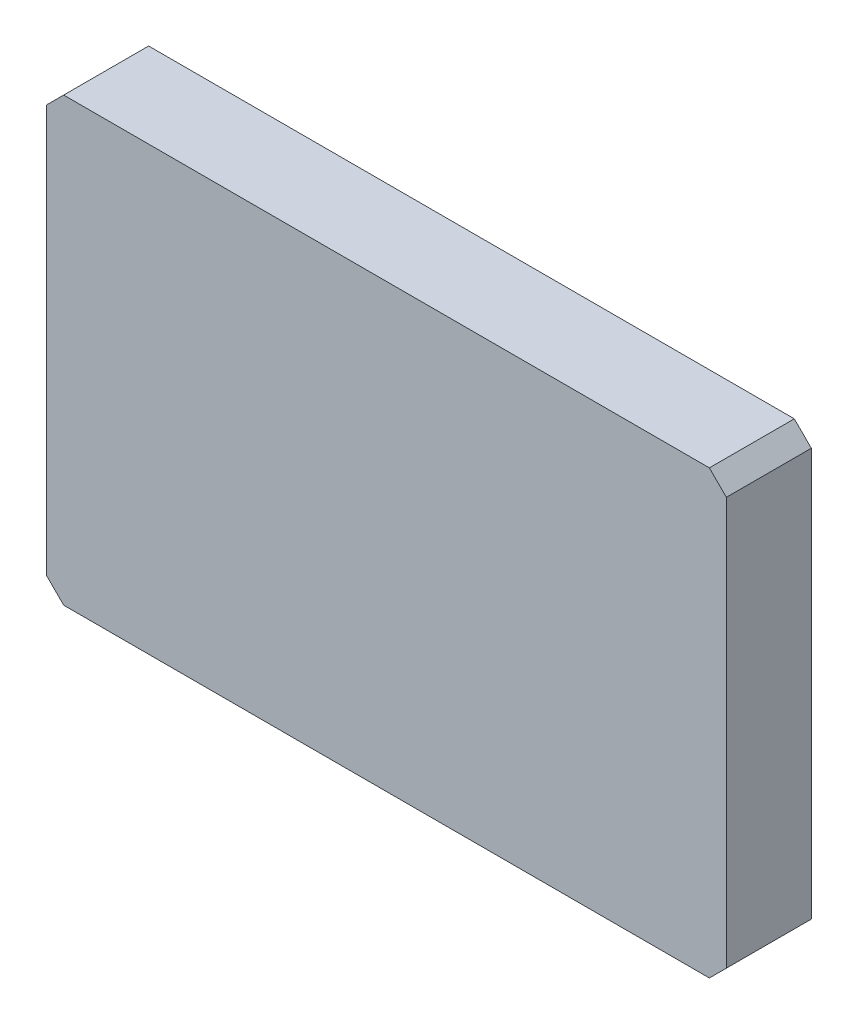
SolidWorks part; units mm, degrees
material "Q235-A "
ref_plane "前视基准面" through (0, 0, 0) normal (0, 0, 1) x (1, 0, 0)
ref_plane "上视基准面" through (0, 0, 0) normal (0, 1, 0) x (1, 0, 0)
ref_plane "右视基准面" through (0, 0, 0) normal (1, 0, 0) x (0, 0, -1)
sketch "草图1" plane through (0, 0, 0) normal (0, 0, 1) x (1, 0, 0)
  line L1 (-100, 65) -> (100, 65)
  line L2 (-100, 65) -> (-100, -65)
  line L3 (-100, -65) -> (100, -65)
  line L4 (100, 65) -> (100, -65)
  line L5 (-100, 65) -> (100, -65) construction
  line L6 (-100, -65) -> (100, 65) construction
  point P0 (0, 0)
  dimension "D1" = 200
  dimension "D2" = 130
extrude "凸台-拉伸1" add sketch "草图1" along normal blind 25
chamfer "倒角1" distance 5 angle 45 4 edges at (-100, -65, 12.5) (100, -65, 12.5) (-100, 65, 12.5) (100, 65, 12.5)
